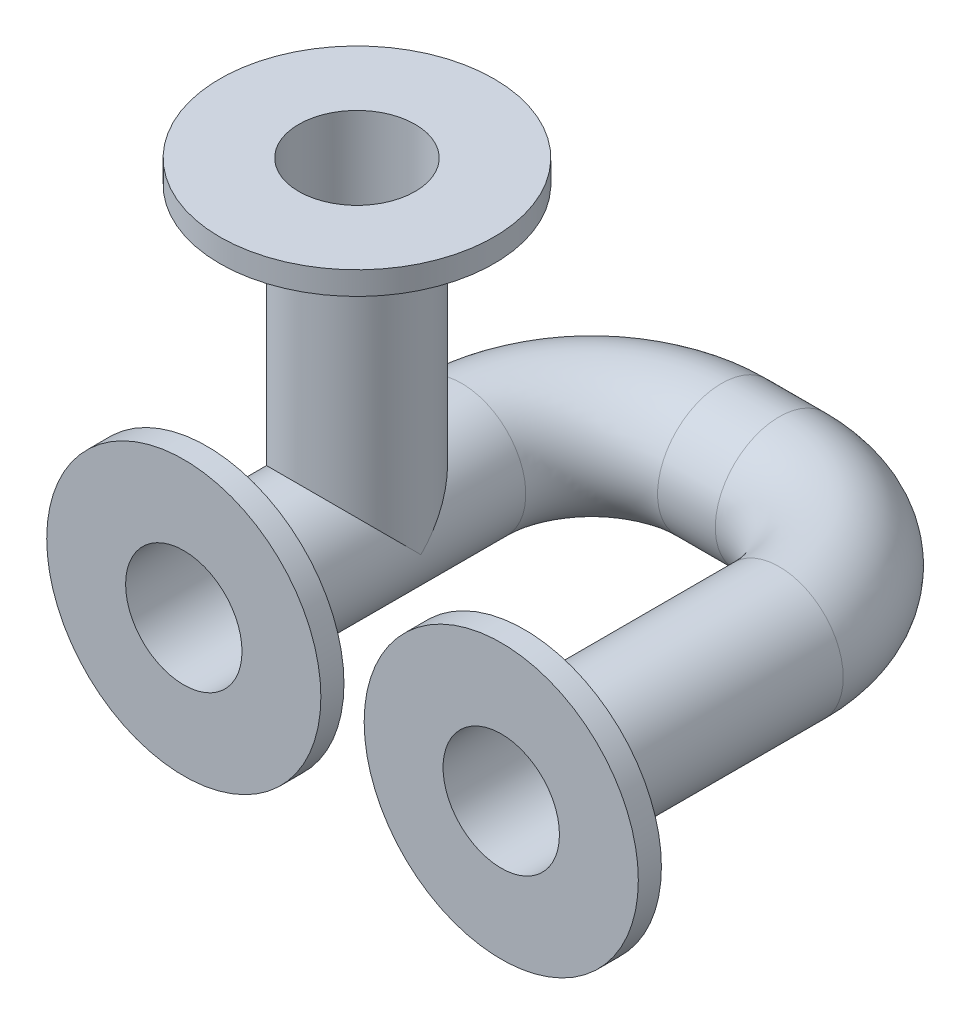
SolidWorks part; units mm, degrees
material "普通碳钢"
ref_plane "Front Plane" through (0, 0, 0) normal (0, 0, 1) x (1, 0, 0)
ref_plane "Top Plane" through (0, 0, 0) normal (0, 1, 0) x (1, 0, 0)
ref_plane "Right Plane" through (0, 0, 0) normal (1, 0, 0) x (0, 0, -1)
sketch "Sketch1" plane through (0, 0, 0) normal (0, 0, 1) x (1, 0, 0)
  circle A0 centre (0, 0) radius 66.5
  circle A1 centre (0, 0) radius 60.5
  dimension "D1" = 133
  dimension "D2" = 6
sketch "Sketch2" plane through (0, 0, 0) normal (0, 1, 0) x (1, 0, 0)
  line L0 (0, 0) -> (0, 265)
  line L1 (135, 400) -> (195, 400)
  line L2 (330, 265) -> (330, 0)
  arc A0 (195, 400) -> (330, 265) centre (195, 265) cw
  arc A1 (0, 265) -> (135, 400) centre (135, 265) cw
  point P9 (0, 400)
  dimension "D3" = 135
  dimension "D1" = 330
  dimension "D2" = 400
sweep "Sweep1" add profiles "Sketch1" path "Sketch2"
sketch "Sketch3" plane through (0, 0, 0) normal (0, 0, 1) x (1, 0, 0)
  circle A0 centre (330, 0) radius 60.5
  circle A1 centre (330, 0) radius 142.5
  circle A2 centre (0, 0) radius 60.5
  circle A3 centre (0, 0) radius 142.5
  dimension "D1" = 285
  dimension "D2" = 285
extrude "Boss-Extrude1" add sketch "Sketch3" along normal blind 24
sketch "Sketch4" plane through (0, 0, 0) normal (0, 1, 0) x (1, 0, 0)
  line L0 (-142.5, -24) -> (142.5, -24) construction
  circle A0 centre (0, 156) radius 66.5
  circle A1 centre (0, 156) radius 60.5
  dimension "D1" = 133
  dimension "D2" = 6
  dimension "D3" = 180
extrude "Boss-Extrude2" add sketch "Sketch4" along normal blind 300
sketch "Sketch5" plane through (0, 300, 0) normal (0, 1, 0) x (1, 0, 0)
  circle A0 centre (0, 156) radius 142.5
  circle A1 centre (0, 156) radius 60.5
  dimension "D1" = 285
extrude "Boss-Extrude3" add sketch "Sketch5" along normal blind 24
